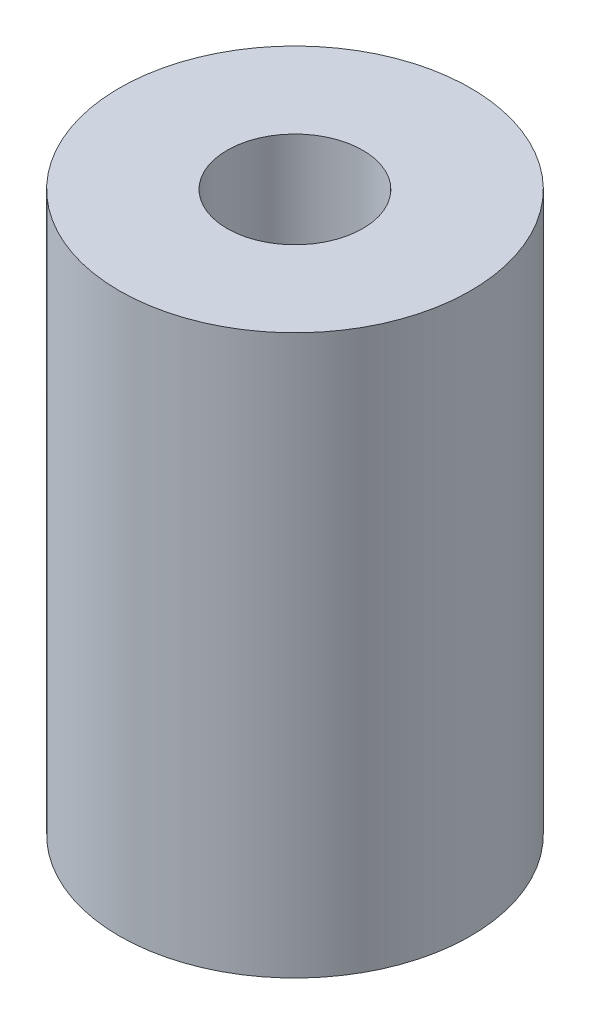
SolidWorks part; units mm, degrees
material "SS400B"
ref_plane "Front Plane" through (0, 0, 0) normal (0, 0, 1) x (1, 0, 0)
ref_plane "Top Plane" through (0, 0, 0) normal (0, 1, 0) x (1, 0, 0)
ref_plane "Right Plane" through (0, 0, 0) normal (1, 0, 0) x (0, 0, -1)
sketch "Sketch1" plane through (0, 0, 0) normal (0, 1, 0) x (1, 0, 0)
  circle A0 centre (0, 0) radius 11
  dimension "D1" = 22
extrude "Boss-Extrude1" add sketch "Sketch1" along normal blind 35
hole_wizard "M10 Tapped Hole1" positions "Sketch2" profile "Sketch3" tap size "M10" standard "GB" end condition through all
sketch "Sketch2" plane through (0, 35, 0) normal (0, 1, 0) x (1, 0, 0)
  point P0 (0, 0)
sketch "Sketch3" plane through (0, 35, 0) normal (1, 0, 0) x (0, 0, 1)
  line L0 (0, 0) -> (0, 35)
  line L1 (0, 35) -> (4.25, 35)
  line L2 (4.25, 35) -> (4.25, 0)
  line L5 (4.25, 0) -> (0, 0)
  line L11 (0, -6.35) -> (0, 107.95) construction
  dimension "通孔螺纹孔钻头直径" = 8.5
  dimension "通孔螺纹孔钻头深度" = 35
cosmetic thread "Cosmetic Thread1"
